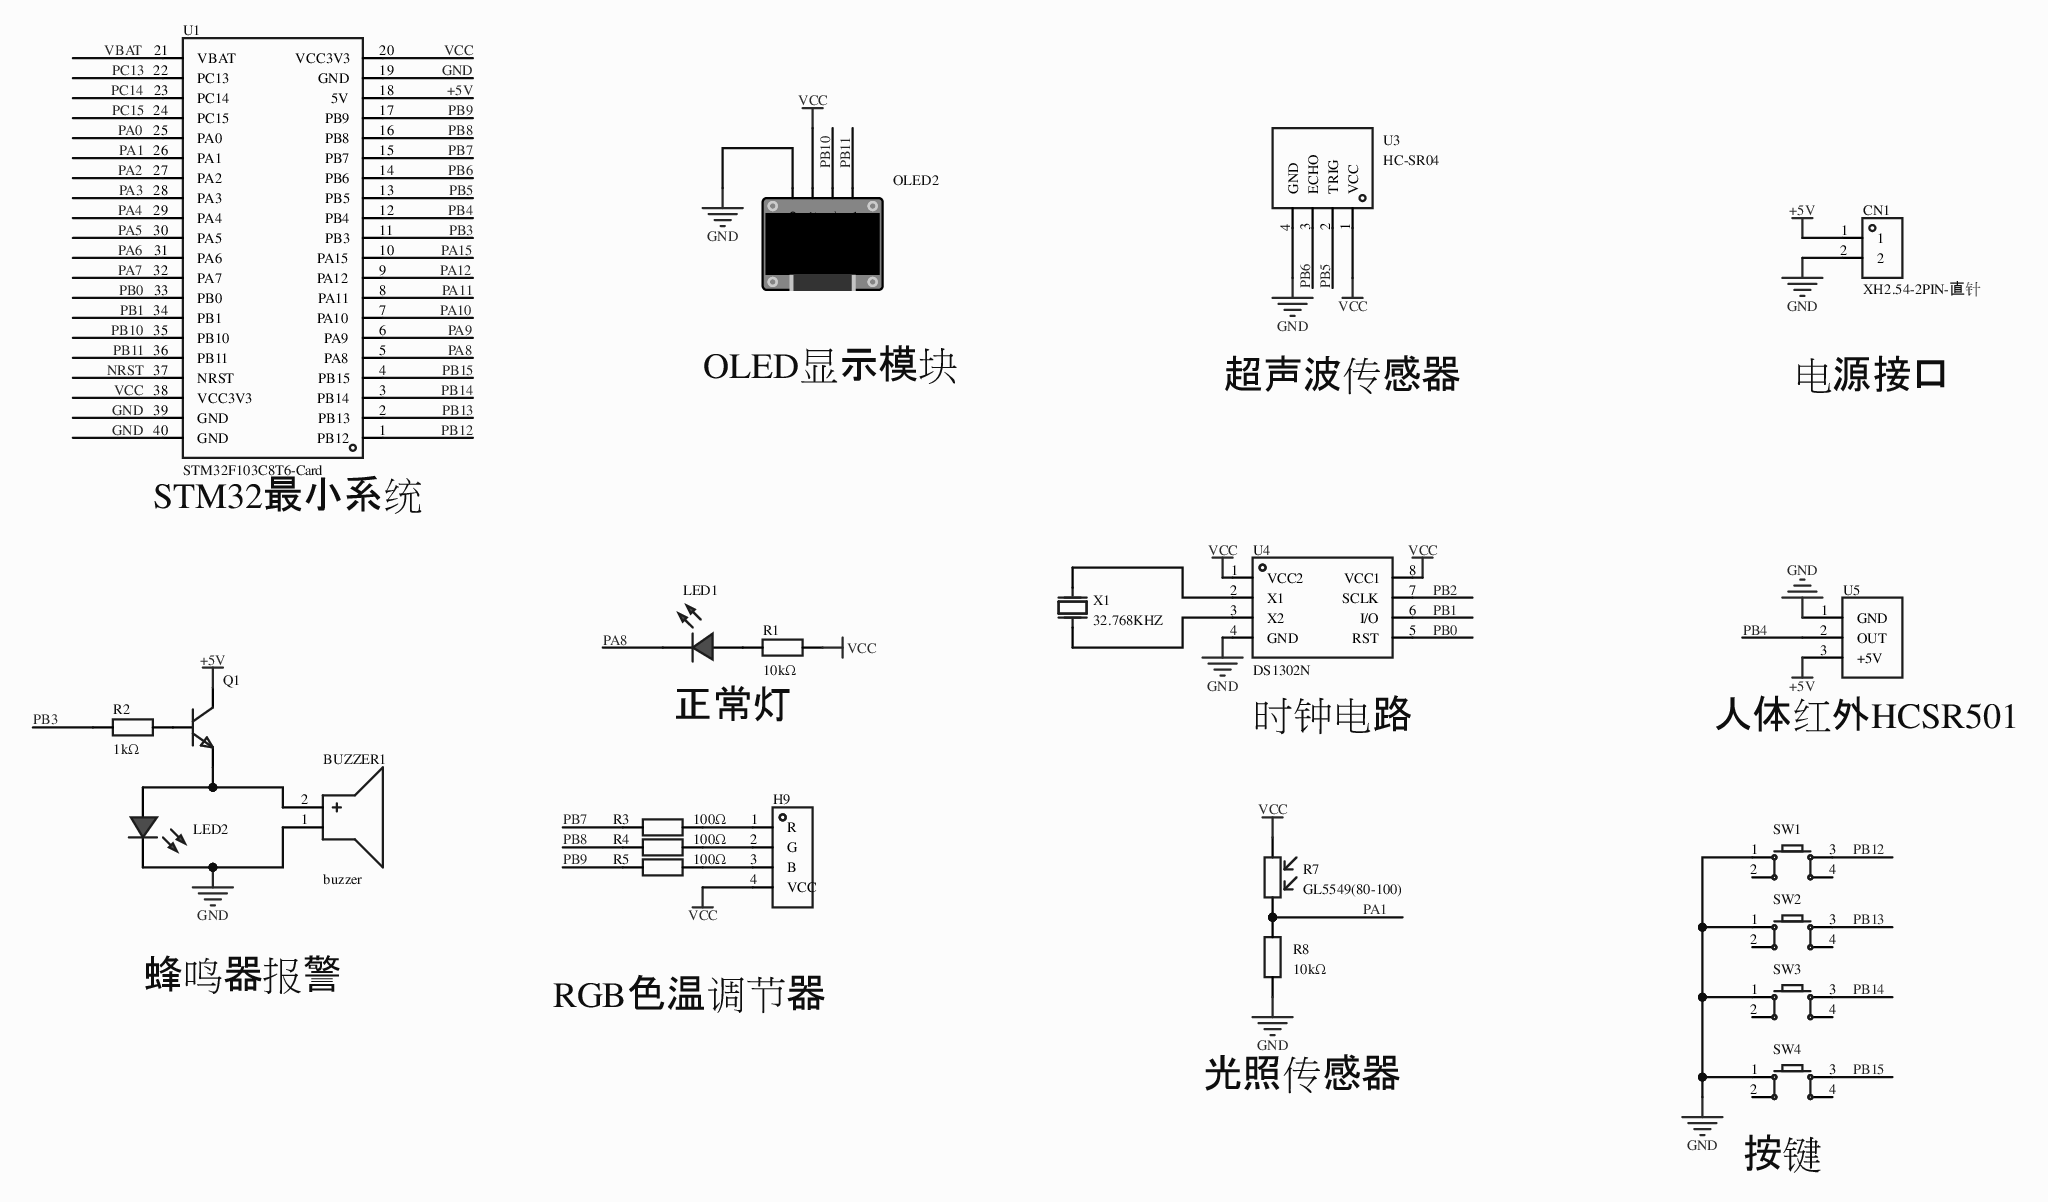
[diagram p0: MISC51867-3.schdoc]
# Altium project MISC51867-2.PrjPcb
1 sheet, 23 parts. Net scope: global (net labels, ports and power ports of the same name join across sheets).
Board file: MISC51867.pcbdoc

## Sheet MISC51867-3.schdoc
size 297 x 209 mm; Version: V1.0; @Project Name: MISC51867; @Page Count: 1; @Update Date: 2026-05-22; @Create Date: 2026-05-22; @Schematic Name: MISC51867; @Page No: 1; @Create Time: 23:22:16; @Update Time: 17:32:40; @Board Name: MISC51867

### Parts
BUZZER1  buzzer  [BUZ-TH_BD12.0-P6.00-D0.9-RD]
CN1  XH2.54-2PIN-直针  [CONN-TH_XH2.54-2P]
H9  (no value)  [HDR-TH_4P-P2.54-V-F]
LED1  (no value)  [LED_TH-3mm]
LED2  (no value)  [LED_TH-3mm]
OLED2  (no value)  [0.96OLED_4P]
Q1  (no value)  [S8050_TO_92]
R1  10kΩ  [Res_1/8W]
R2  1kΩ  [Res_1/8W]
R3  100Ω  [Res_1/8W]
R4  100Ω  [Res_1/8W]
R5  100Ω  [Res_1/8W]
R7  GL5549(80-100)  [RES-TH_L5.1-W4.3-P3.40-D0.5]
R8  10kΩ  [Res_1/8W]
SW1  (no value)  [SW-TH_4P-L6.0-W6.0-P4.50-LS6.5]
SW2  (no value)  [SW-TH_4P-L6.0-W6.0-P4.50-LS6.5]
SW3  (no value)  [SW-TH_4P-L6.0-W6.0-P4.50-LS6.5]
SW4  (no value)  [SW-TH_4P-L6.0-W6.0-P4.50-LS6.5]
U1  STM32F103C8T6-Card  [CONN-TH_L53.3-W22.9_STM32F103C8T6-CARD]
U3  HC-SR04  [TH_HC-SR04V]
U4  DS1302N  [DIP-8_L9.7-W6.4-P2.54-LS7.6-BL]
U5  (no value)  [HC-SR501]
X1  32.768KHZ  [HC-49S_L11.5-W5.0-P4.88]

### Nets
+5V: CN1.1 Q1.3(C) U1.18(5V) U5.3(+5V)
GND: BUZZER1.1(-) CN1.2 LED2.2(A) OLED2.1(GND) R8.1 SW1.1 SW2.1 SW3.1 SW4.1 U1.19(GND) U1.39(GND) U1.40(GND) U3.4(GND) U4.4(GND) U5.1(GND)
VCC: H9.4(VCC) OLED2.2(VCC) R1.2 R7.1 U1.20(VCC3V3) U1.38(VCC3V3) U3.1(VCC) U4.1(VCC2) U4.8(VCC1)
NRST: U1.37(NRST)
PA0: U1.25(PA0)
PA1: R7.2 R8.2 U1.26(PA1)
PA2: U1.27(PA2)
PA3: U1.28(PA3)
PA4: U1.29(PA4)
PA5: U1.30(PA5)
PA6: U1.31(PA6)
PA7: U1.32(PA7)
PA8: LED1.2(A) U1.5(PA8)
PA9: U1.6(PA9)
PA10: U1.7(PA10)
PA11: U1.8(PA11)
PA12: U1.9(PA12)
PA15: U1.10(PA15)
PB0: U1.33(PB0) U4.5(RST)
PB1: U1.34(PB1) U4.6(I/O)
PB2: U4.7(SCLK)
PB3: R2.1 U1.11(PB3)
PB4: U1.12(PB4) U5.2(OUT)
PB5: U1.13(PB5) U3.2(TRIG)
PB6: U1.14(PB6) U3.3(ECHO)
PB7: R3.1 U1.15(PB7)
PB8: R4.1 U1.16(PB8)
PB9: R5.1 U1.17(PB9)
PB10: OLED2.3(SCL) U1.35(PB10)
PB11: OLED2.4(SDA) U1.36(PB11)
PB12: SW1.3 U1.1(PB12)
PB13: SW2.3 U1.2(PB13)
PB14: SW3.3 U1.3(PB14)
PB15: SW4.3 U1.4(PB15)
PC13: U1.22(PC13)
PC14: U1.23(PC14)
PC15: U1.24(PC15)
VBAT: U1.21(VBAT)
NetBUZZER1_2: BUZZER1.2(+) LED2.1(C) Q1.1(E)
NetH9_1: H9.1(R) R3.2
NetH9_2: H9.2(G) R4.2
NetH9_3: H9.3(B) R5.2
NetLED1_1: LED1.1(C) R1.1
NetQ1_2: Q1.2(B) R2.2
NetU4_2: U4.2(X1) X1.2(OSC2)
NetU4_3: U4.3(X2) X1.1(OSC1)

Not connected (* = marked no-connect by the designer): SW1 2 4; SW2 2 4; SW3 2 4; SW4 2 4

### Notes on the sheet
- OLED显示模块
- 超声波传感器
- 电源接口
- (near U1) STM32最小系统
- 正常灯
- (near U4) 时钟电路
- (near U5) 人体红外HCSR501
- 蜂鸣器报警
- RGB色温调节器
- 光照传感器
- (near SW4) 按键

### Library data of the parts
BUZZER1 = buzzer: AddInBom: yes; ModelId: af17e4151ed84fc2a628230bf23763630819f05c4eef4c71ace90d822a990e87; ModelTransform: 472.44,472.176,0,270,0,0,0,0,-196.85; Symbol: BUZZER; Device: buzzer; LCSC Part Name: buzzer; SupplierPart: C9900014030; ManufacturerPart: buzzer; Supplier Footprint: buzzer; JLCPCB Part Class: Extended Part; Supplier: LCSC; ConvertToPcb: yes; FootprintName: BUZ-TH_BD12.0-P6.00-D0.9-RD; ModelName: BUZ-TH_BD12.0-P6.00-D0.9-RD
CN1 = XH2.54-2PIN-直针: AddInBom: yes; ModelId: c3cc11bd8b8748c1ae6bc231aac3a1ff0819f05c4eef4c71ace90d822a990e87; ModelTransform: 296.889,230.315,0,0,0,0,0,26.653,-137.795; Symbol: XH2.54-2PIN-直针; Device: XH2.54-2PIN-直针; LCSC Part Name: XH2.54-2PIN-直针; SupplierPart: C9900011425; ManufacturerPart: XH2.54-2PIN-直针; Supplier Footprint: XH2.54-2PIN; JLCPCB Part Class: Extended Part; Supplier: LCSC; ConvertToPcb: yes; FootprintName: CONN-TH_XH2.54-2P; ModelName: CONN-TH_XH2.54-2P
H9 = HDR-F_2.54_1x4P: Symbol: 2.54-1*4P母_1; ConvertToPcb: yes; ModelId: d187812051054f85879fcaa51a310d8e0819f05c4eef4c71ace90d822a990e87; ModelTransform: 419.6842,98.464,0,0,0,0,0,0,-118.11; Device: HDR-F_2.54_1x4P; AddInBom: yes; SupplierPart: C2718488; Supplier Footprint: 插件; FootprintName: HDR-TH_4P-P2.54-V-F; ModelName: HDR-TH_4P-P2.54-V-F
LED1 LED2 = LED_TH-R_3mm: 3D Model: a497c992633541038a38947cdc58012f0819f05c4eef4c71ace90d822a990e87; 3D Model Transform: 141.274,153.327,0,0,0,0,-5.984,0,-137.795; ConvertToPcb: yes; ModelName: LED-TH-3mm_R; Symbol: LED_TH-R; Device: LED_TH-R_3mm; Supplier Footprint: 插件; AddInBom: yes; FootprintName: LED_TH-3mm
OLED2 = 0.96OLED模块_4P: ConvertToPcb: yes; ModelId: 79c000fdb68d45a296c2e9bedf4f9055; ModelTransform: 1393.69792,1318.895,0,0,0,0,0,-560.079,-137.795; Symbol: 0.96OLED模块_4P; Device: 0.96OLED模块_4P; AddInBom: yes; FootprintName: 0.96OLED_4P; Supplier Footprint: 插件; ModelName: 0.96OLED_4P
Q1 = S8050_TO_NPN: ConvertToPcb: yes; ModelId: aafe8e06f2154e7c93506efd0d6632dd; ModelName: TO-92-3_L4.9-W3.7-P1.27-L; ModelTransform: 180.78,141.44,417.3,0,0,0,0,0,-200; Symbol: S8050_TO_NPN; Device: S8050_TO_NPN; AddInBom: yes; Supplier Footprint: TO-92; FootprintName: S8050_TO_92
R1 = Res_AXIAL-1/8W: Symbol: 电阻; ConvertToPcb: yes; ModelId: b2b5ae7ae4c642178fe0039925c86a3f0819f05c4eef4c71ace90d822a990e87; ModelName: RES-TH_BD1.8-L3.2-P7.20-D0.4; ModelTransform: 282.86,66.88,253.09,0,0,0,0,0,-191; Device: Res_AXIAL-1/8W; AddInBom: yes; Supplier Footprint: 轴向引线; Value: 10kΩ; FootprintName: Res_1/8W
R2-R5 R8 = Res_AXIAL-1/8W: Symbol: 电阻; 3D Model: b2b5ae7ae4c642178fe0039925c86a3f0819f05c4eef4c71ace90d822a990e87; 3D Model Transform: 282.86,66.88,253.09,0,0,0,0,0,-191; ConvertToPcb: yes; ModelName: RES-TH_BD1.8-L3.2-P7.20-D0.4; Device: Res_AXIAL-1/8W; Supplier Footprint: 轴向引线; AddInBom: yes; FootprintName: Res_1/8W
  R2: Value: 1kΩ
  R3-R5: Value: 100Ω
  R8: Value: 10kΩ
R7 = GL5549(80-100): 暗电阻:20MΩ;亮电阻@10Lux:80kΩ~150kΩ;光谱峰值(波长):540nm;; Manufacturer: JCHL(晶创和立); AddInBom: yes; ModelId: cb75fcf2d6c94cac811f2579121b87200819f05c4eef4c71ace90d822a990e87; ModelTransform: 169.291,200.39669,0,0,0,0,-3.937,0,-137.795; Dark Resistance: 20MΩ; Voltage - Max: 150V; Wavelength - Peak: 540nm; γ Value: 0.8; Pitch: 3.4mm; Symbol: GL5549(80-100); Device: GL5549(80-100); LCSC Part Name: 光敏电阻性能参数; SupplierPart: C10078; ManufacturerPart: GL5549(80-100); Supplier Footprint: 插件,P=3.4mm; JLCPCB Part Class: Extended Part; Datasheet: https://item.szlcsc.com/datasheet/GL5549(80-100)/10617.html; Supplier: LCSC; ConvertToPcb: yes; FootprintName: RES-TH_L5.1-W4.3-P3.40-D0.5; ModelName: RES-TH_L5.1-W4.3-P3.40-D0.5; Cell Resistance @ Illuminance: 80kΩ~150kΩ; Operating Temperature: -30℃~+70℃; Length: 5.1mm; Width: 4.3mm; Height: 2.4mm
SW1-SW4 = Key_TH_6x6x6: 触点电流:50mA;额定电压(DC):12V;绝缘电阻:100MΩ;电路结构:单刀单掷;安装方式:直插;按钮形状:圆形按钮;按钮/盖帽颜色:黑色;作用力:260gf@±30gf;工作温度:-25℃~+70℃;引脚样式:PC引脚;开关长度:6mm;开关宽度:6mm;开关高度:6mm;带支架:否;; Symbol: 轻触按键; AddInBom: yes; ModelId: 20eee248bc684ccd8cbdbb1d0d91ec6f0819f05c4eef4c71ace90d822a990e87; ModelName: SW-TH_4P-L6.0-W6.0-H5.0-LS6.5-P4.50; ModelTransform: 236.22,323.03,0,90,0,0,0,0,-137.795; Device: Key_TH_6x6x6; FootprintName: SW-TH_4P-L6.0-W6.0-P4.50-LS6.5; ConvertToPcb: yes; Supplier Footprint: 插件
U1 = STM32F103C8T6-Card: AddInBom: yes; Device: STM32F103C8T6-Card; Symbol: STM32F103C8T6-CARD; FootprintName: CONN-TH_L53.3-W22.9_STM32F103C8T6-CARD; LCSC Part Name: STM32F103C8T6-Card; SupplierPart: C9900077949; ManufacturerPart: STM32F103C8T6-Card; Supplier Footprint: 插件; Supplier: LCSC; ConvertToPcb: yes
U3 = HC-SR04: Manufacturer: Universal Microelectronics; AddInBom: yes; Symbol: HC-SR04; Device: HC-SR04; LCSC Part Name: HC-SR04; SupplierPart: C19857336; ManufacturerPart: HC-SR04; Supplier Footprint: -; JLCPCB Part Class: 扩展库; Datasheet: https://atta.szlcsc.com/upload/public/pdf/source/20240122/47B8E374E428935B7962A2189EF91AAC.pdf; Supplier: LCSC; ConvertToPcb: yes; FootprintName: TH_HC-SR04V
U4 = DS1302N: Manufacturer: HGSEMI(华冠); AddInBom: yes; ModelId: 5746b540d01a4d1b9eb6b4f989297bc70819f05c4eef4c71ace90d822a990e87; ModelName: DIP-8_L9.8-W6.6-H3.5-LS7.62-P2.54; ModelTransform: 385.826,311.8104,0,0,0,0,0,0,-118.11; Voltage - Supply: 2V~5.5V; Symbol: DS1302N; Device: DS1302N; LCSC Part Name: DS1302N; SupplierPart: C398065; ManufacturerPart: DS1302N; Supplier Footprint: DIP-8; JLCPCB Part Class: Extended Part; Datasheet: https://item.szlcsc.com/datasheet/DS1302N/379831.html; Supplier: LCSC; ConvertToPcb: yes; FootprintName: DIP-8_L9.7-W6.4-P2.54-LS7.6-BL; Operating Temperature: 0℃~+70℃
U5 = HCSR501: AddInBom: yes; ModelId: 94ce8706d57546399d41295b6bf7cf3f6d41313a9ef5454fad103a4ed4b4dcb7; ModelTransform: 1287.39901,980.3129697240615,956.6909550732486,0,90,0,23.62205,472.44094,196.85039; Symbol: HCSR501; Device: HCSR501; ConvertToPcb: yes; ModelName: hc-sr501; FootprintName: HC-SR501
X1 = 8MHZ: Symbol: 8MHZ_C9900021358; AddInBom: yes; ModelId: 0135de1822fc414cabce320cefc215fe0819f05c4eef4c71ace90d822a990e87; ModelTransform: 452.08264,196.85,0,0,0,0,0,0,-196.85; Device: 8MHZ; Manufacturer Part: 32.768KHZ; LCSC Part Name: 8MHZ; SupplierPart: C9900021358; Supplier Footprint: X-HC49U直插; JLCPCB Part Class: Extended Part; Supplier: LCSC; ConvertToPcb: yes; FootprintName: HC-49S_L11.5-W5.0-P4.88; ModelName: HC-49S_L11.5-W5.0-P4.88